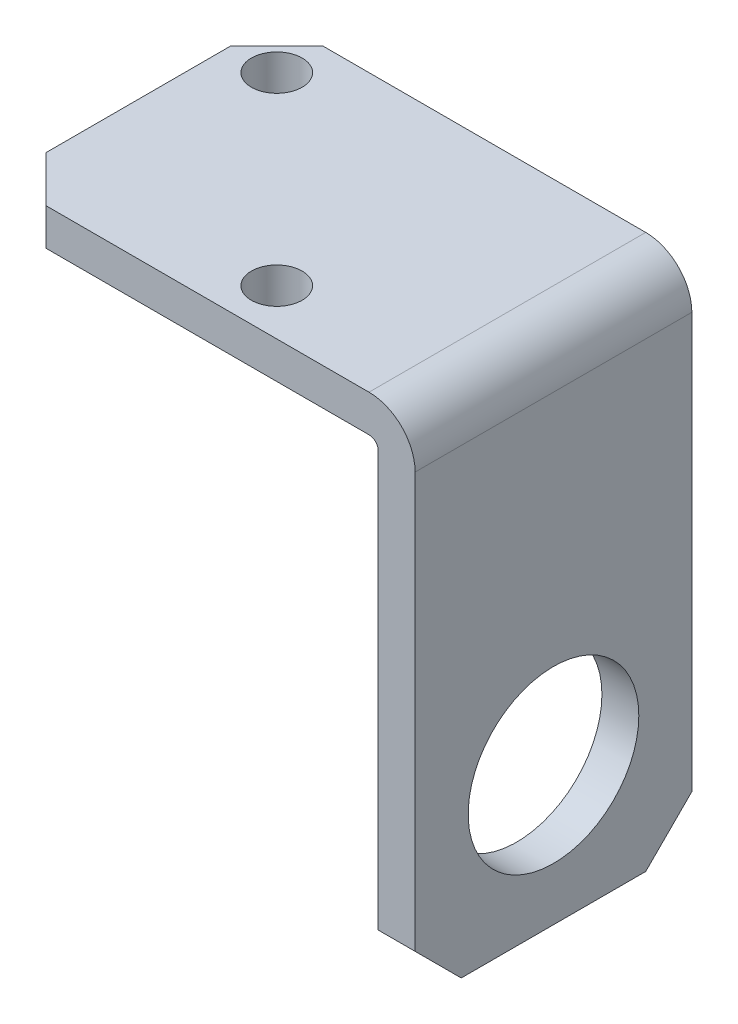
SolidWorks part; units mm, degrees
material "1023 碳钢板 (SS)"
ref_plane "前视基准面" through (0, 0, 0) normal (0, 0, 1) x (1, 0, 0)
ref_plane "上视基准面" through (0, 0, 0) normal (0, 1, 0) x (1, 0, 0)
ref_plane "右视基准面" through (0, 0, 0) normal (1, 0, 0) x (0, 0, -1)
sketch "草图1" plane through (0, 0, 0) normal (0, 0, 1) x (1, 0, 0)
  line L0 (0, 0) -> (40, 0)
  line L1 (45, -5) -> (45, -55)
  line L2 (0, -4) -> (40, -4)
  line L3 (41, -5) -> (41, -55)
  line L4 (0, 0) -> (0, -4)
  line L5 (45, -55) -> (41, -55)
  arc A0 (40, 0) -> (45, -5) centre (40, -5) cw
  arc A1 (40, -4) -> (41, -5) centre (40, -5) cw
  point P6 (45, 0)
  dimension "D3" = 5
  dimension "D1" = 55
  dimension "D2" = 45
  dimension "D4" = 4
extrude "凸台-拉伸1" add sketch "草图1" along normal blind 30 contours L5 L3 A1 L2 L4 L0 A0 L1
sketch "草图3" plane through (45, 0, 0) normal (1, 0, 0) x (0, 0, -1)
  line L0 (-30, -55) -> (0, -55) construction
  circle A0 centre (-15, -40) radius 9.25
  dimension "D1" = 18.5
  dimension "D2" = 15
extrude "切除-拉伸1" cut sketch "草图3" against normal blind 30
sketch "草图4" plane through (0, 0, 0) normal (0, 1, 0) x (1, 0, 0)
  line L0 (0, -30) -> (40, -30) construction
  line L1 (0, -30) -> (0, 0) construction
  circle A0 centre (5, -5) radius 2.75
  circle A1 centre (25, -25) radius 2.75
  dimension "D3" = 5.5
  dimension "D4" = 5
  dimension "D5" = 5.5
  dimension "D6" = 20
  dimension "D1" = 20
  dimension "D2" = 5
extrude "切除-拉伸2" cut sketch "草图4" against normal blind 30
chamfer "倒角1" distance 5 angle 45 4 edges at (43, -55, 0) (43, -55, 30) (0, -2, 0) (0, -2, 30)
